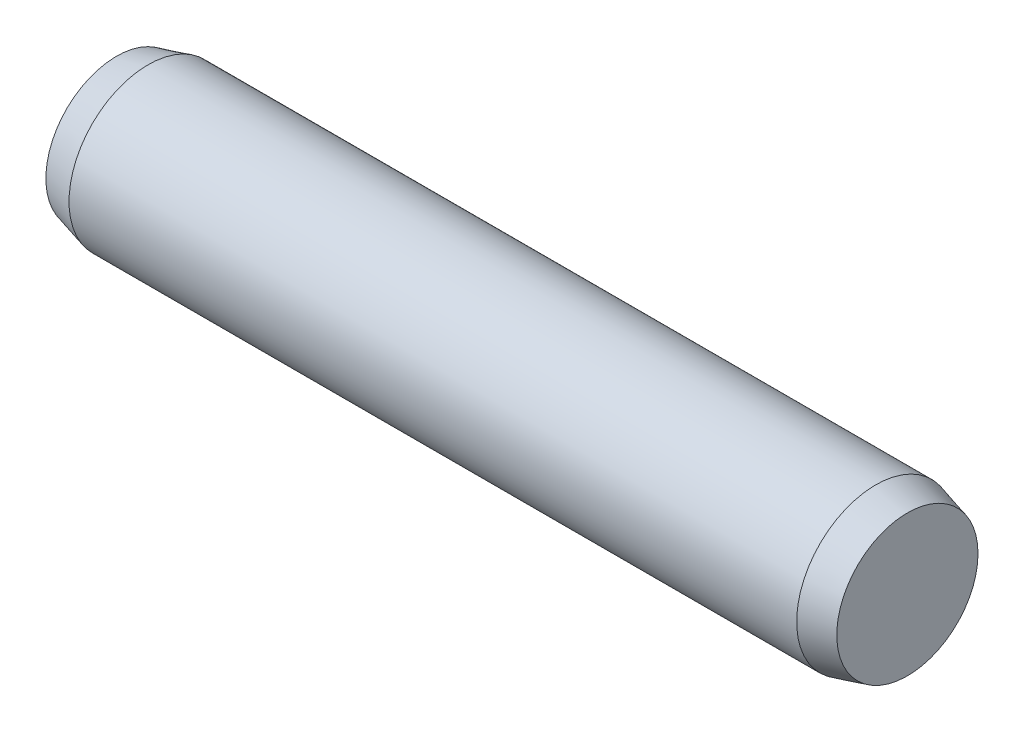
from build123d import *


with BuildPart() as part:
    # Dimensioned Sketch → Base-Revolve (revolve)
    with BuildSketch(Plane.XY, mode=Mode.PRIVATE) as base_revolve_sk:
        Polygon((0, 0), (40, 0), (40, 3.571281292), (38.4, 4), (1.6, 4), (0, 3.571281292), align=None)
    revolve(base_revolve_sk.sketch.rotate(Axis((0, 0, 0), (-1, 0, 0)), 90), axis=Axis((0, 0, 0), (-1, 0, 0)))


solid = part.part
